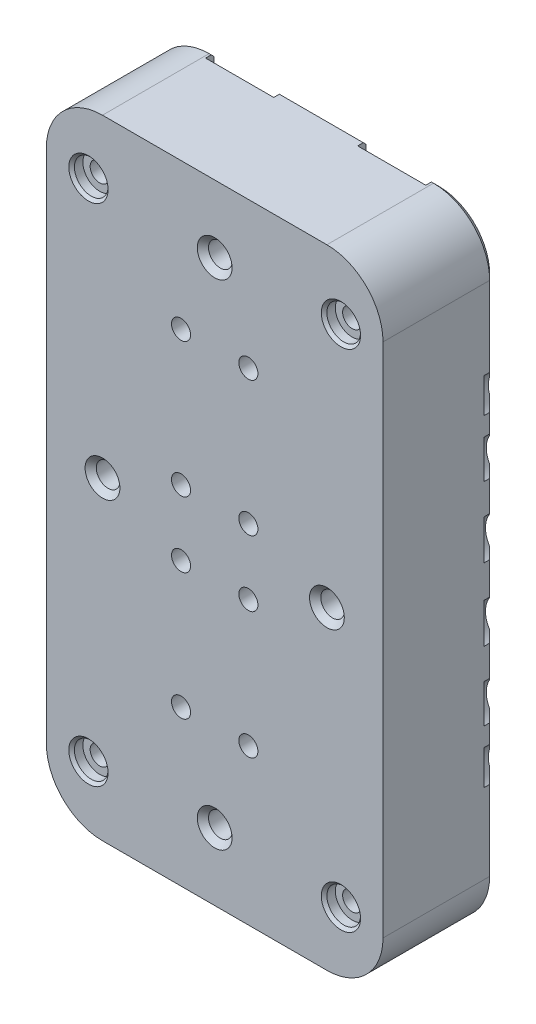
SolidWorks part; units mm, degrees
material "POM 乙缩醛共聚物"
ref_plane "前视" through (0, 0, 0) normal (0, 0, 1) x (1, 0, 0)
ref_plane "上视" through (0, 0, 0) normal (0, 1, 0) x (1, 0, 0)
ref_plane "右视" through (0, 0, 0) normal (1, 0, 0) x (0, 0, -1)
sketch "草图1" plane through (0, 0, 0) normal (0, 0, 1) x (1, 0, 0)
  line L0 (-30, 46) -> (-30, -46)
  line L1 (-20, -56) -> (20, -56)
  line L2 (30, -46) -> (30, 46)
  line L3 (20, 56) -> (-20, 56)
  line L4 (-30, 0) -> (0, 0) construction
  line L5 (0, 56) -> (0, 0) construction
  arc A0 (-30, -46) -> (-20, -56) centre (-20, -46) ccw
  arc A1 (20, -56) -> (30, -46) centre (20, -46) ccw
  arc A2 (30, 46) -> (20, 56) centre (20, 46) ccw
  arc A3 (-30, 46) -> (-20, 56) centre (-20, 46) cw
  dimension "D1" = 10
  dimension "D2" = 112
  dimension "D3" = 60
extrude "凸台-拉伸1" add sketch "草图1" along normal blind 20
hole_wizard "M4 螺纹孔1" positions "草图2" profile "草图3" tap size "M4" standard "AS" end condition through all
sketch "草图2" plane through (0, 0, 20) normal (0, 0, 1) x (1, 0, 0)
  point P0 (22.5, -45)
  point P3 (-22.5, -45)
  point P6 (-22.5, 45)
  point P9 (22.5, 45)
  point P12 (-112.3936, 267.4308)
sketch "草图3" plane through (22.5, -45, 20) normal (1, 0, 0) x (0, -1, 0)
  line L0 (0, 0) -> (0, 20)
  line L1 (0, 20) -> (1.65, 20)
  line L2 (1.65, 20) -> (1.65, 0)
  line L5 (1.65, 0) -> (0, 0)
  line L11 (0, -6.35) -> (0, 107.95) construction
  dimension "通孔螺纹孔钻头直径" = 3.3
  dimension "通孔螺纹孔钻头深度" = 20
cosmetic thread "孔螺蚊线1" parameters "D2"=4
cosmetic thread "孔螺蚊线2" parameters "D2"=4
cosmetic thread "孔螺蚊线6" parameters "D2"=4
cosmetic thread "孔螺蚊线19" parameters "D2"=4
sketch "草图4" plane through (0, 0, 20) normal (0, 0, 1) x (1, 0, 0)
  circle A0 centre (22.5, -45) radius 3
  circle A1 centre (-22.5, -45) radius 3
  circle A2 centre (22.5, 45) radius 3
  circle A3 centre (-22.5, 45) radius 3
  dimension "D1" = 6
  dimension "D2" = 6
  dimension "D3" = 6
  dimension "D4" = 6
extrude "切除-拉伸1" cut sketch "草图4" against normal blind 2
hole_wizard "大小六角凹头盖螺钉柱孔0" positions "草图6" profile "草图7" counterbore size "M3" standard "AS" end condition through all
sketch "草图6" plane through (0, 0, 0) normal (0, 0, -1) x (-1, 0, 0)
  circle A0 centre (22.5, -45) radius 1.65 construction
  point P0 (22.5, 45)
  point P6 (-22.5, -45)
  point P9 (-22.5, 45)
  point P12 (22.5, -45)
sketch "草图7" plane through (-22.5, 45, 0) normal (1, 0, 0) x (0, 1, 0)
  line L0 (0, 0) -> (0, 20)
  line L1 (0, 20) -> (1.7, 20)
  line L3 (1.7, 20) -> (1.7, 4)
  line L4 (1.7, 4) -> (3, 4)
  line L5 (3, 4) -> (3, 0)
  line L7 (3, 0) -> (0, 0)
  line L11 (0, -6.35) -> (0, 107.95) construction
  dimension "通孔孔直径" = 3.4
  dimension "通孔孔深度" = 20
  dimension "柱形沉头孔直径" = 6
  dimension "柱形沉头孔深度" = 4
hole_wizard "大小六角凹头盖螺钉柱孔0" positions "草图10" profile "草图11" counterbore size "M3" standard "AS" end condition through all
sketch "草图10" plane through (0, 0, 0) normal (0, 0, -1) x (-1, 0, 0)
  point P0 (6, 5.95)
  point P7 (-6, 5.95)
  point P13 (6, 29.95)
  point P16 (-6, 29.95)
sketch "草图11" plane through (-6, 5.95, 0) normal (1, 0, 0) x (0, 1, 0)
  line L0 (0, 0) -> (0, 20)
  line L1 (0, 20) -> (1.7, 20)
  line L3 (1.7, 20) -> (1.7, 4)
  line L4 (1.7, 4) -> (3, 4)
  line L5 (3, 4) -> (3, 0)
  line L7 (3, 0) -> (0, 0)
  line L11 (0, -6.35) -> (0, 107.95) construction
  dimension "通孔孔直径" = 3.4
  dimension "通孔孔深度" = 20
  dimension "柱形沉头孔直径" = 6
  dimension "柱形沉头孔深度" = 4
hole_wizard "大小六角凹头盖螺钉柱孔2" positions "草图13" profile "草图14" counterbore size "M3" standard "AS" end condition through all
sketch "草图13" plane through (0, 0, 0) normal (0, 0, -1) x (-1, 0, 0)
  point P0 (-6, -5.75)
  point P3 (6, -5.75)
  point P6 (-6, -28.35)
  point P9 (6, -28.35)
sketch "草图14" plane through (6, -5.75, 0) normal (1, 0, 0) x (0, 1, 0)
  line L0 (0, 0) -> (0, 20)
  line L1 (0, 20) -> (1.7, 20)
  line L3 (1.7, 20) -> (1.7, 4)
  line L4 (1.7, 4) -> (3, 4)
  line L5 (3, 4) -> (3, 0)
  line L7 (3, 0) -> (0, 0)
  line L11 (0, -6.35) -> (0, 107.95) construction
  dimension "通孔孔直径" = 3.4
  dimension "通孔孔深度" = 20
  dimension "柱形沉头孔直径" = 6
  dimension "柱形沉头孔深度" = 4
sketch "草图15" plane through (0, 0, 0) normal (0, 0, 1) x (1, 0, 0)
  line L0 (-20, -56) -> (20, -56) construction
  line L1 (30, -46) -> (30, 46) construction
  line L2 (20, 56) -> (-20, 56) construction
  circle A0 centre (0, -44) radius 6.5
  circle A1 centre (0, 44) radius 6.5
  dimension "D1" = 13
  dimension "D2" = 12
  dimension "D3" = 30
  dimension "D4" = 13
  dimension "D5" = 12
  dimension "D6" = 30
extrude "切除-拉伸3" cut sketch "草图15" along normal blind 8.5
sketch "草图16" plane through (0, 0, 0) normal (0, 0, -1) x (-1, 0, 0)
  circle A0 centre (-20, -0.0001) radius 6.5
  circle A1 centre (20, -0.0001) radius 6.5
  dimension "D1" = 13
  dimension "D2" = 13
  dimension "D3" = 20
  dimension "D4" = 20
extrude "切除-拉伸4" cut sketch "草图16" against normal blind 8.5
hole_wizard "M4 螺纹孔2" positions "草图18" profile "草图19" tap size "M4" standard "AS" end condition through all
sketch "草图18" plane through (0, 0, 8.5) normal (0, 0, -1) x (-1, 0, 0)
  point P0 (-20, -0.0001)
  point P3 (20, -0.0001)
  point P6 (0, 44)
  point P9 (0, -44)
sketch "草图19" plane through (20, -0.0001, 8.5) normal (1, 0, 0) x (0, 1, 0)
  line L0 (0, 0) -> (0, 11.5)
  line L1 (0, 11.5) -> (1.65, 11.5)
  line L2 (1.65, 11.5) -> (1.65, 0)
  line L5 (1.65, 0) -> (0, 0)
  line L11 (0, -6.35) -> (0, 107.95) construction
  dimension "通孔螺纹孔钻头直径" = 3.3
  dimension "通孔螺纹孔钻头深度" = 11.5
cosmetic thread "孔螺蚊线11" parameters "D2"=4
cosmetic thread "孔螺蚊线12" parameters "D2"=4
cosmetic thread "孔螺蚊线13" parameters "D2"=4
cosmetic thread "孔螺蚊线14" parameters "D2"=4
hole_wizard "M5 螺纹孔2" positions "草图20" profile "草图22" tap size "M5" standard "AS"
sketch "草图20" plane through (0, 0, 20) normal (0, 0, 1) x (1, 0, 0)
  point P4 (20, -0.0001)
  point P7 (-20, -0.0001)
  point P10 (0, 44)
  point P13 (0, -44)
sketch "草图22" plane through (20, -0.0001, 20) normal (1, 0, 0) x (0, -1, 0)
  line L0 (0, 0) -> (0, 8.2618)
  line L1 (0, 8.2618) -> (2.1, 7)
  line L2 (2.1, 7) -> (2.1, 0)
  line L5 (2.1, 0) -> (0, 0)
  line L10 (0, 8.2618) -> (-2.1, 7) construction
  line L11 (0, -6.35) -> (0, 107.95) construction
  dimension "螺纹孔钻头直径" = 4.2
  dimension "螺纹孔钻头深度" = 7
  dimension "导头角度" = 118
cosmetic thread "孔螺蚊线15" parameters "D1"=7, "D2"=5
cosmetic thread "孔螺蚊线16" parameters "D1"=7, "D2"=5
cosmetic thread "孔螺蚊线17" parameters "D1"=7, "D2"=5
cosmetic thread "孔螺蚊线18" parameters "D1"=7, "D2"=5
chamfer "倒角1" distance 1 angle 45 8 edges at (30, 0, 0) (27.0711, 53.0711, 0) (27.0711, -53.0711, 0) (0, 56, 0) (0, -56, 0) (-27.0711, 53.0711, 0) (-27.0711, -53.0711, 0) (-30, 0, 0)
sketch "草图23" plane through (0, 0, 0) normal (0, 0, -1) x (-1, 0, 0)
  line L0 (0, 0) -> (33.1344, 0) construction
  line L1 (0, 0) -> (0, -60.1074) construction
  arc A0 (-22.3238, -27.3351) -> (-14.2455, -26.2908) centre (-18.0393, -28.7109) ccw
  arc A1 (-14.2455, -26.2908) -> (-22.3238, -27.3351) centre (-18.53, -24.915) ccw
  arc A2 (14.2455, -26.2908) -> (22.3238, -27.3351) centre (18.53, -24.915) cw
  arc A3 (22.3238, -27.3351) -> (14.2455, -26.2908) centre (18.0393, -28.7109) cw
  arc A4 (22.3238, 27.3351) -> (14.2455, 26.2908) centre (18.0393, 28.7109) ccw
  arc A5 (14.2455, 26.2908) -> (22.3238, 27.3351) centre (18.53, 24.915) ccw
  arc A6 (-14.2455, 26.2908) -> (-22.3238, 27.3351) centre (-18.53, 24.915) cw
  arc A7 (-22.3238, 27.3351) -> (-14.2455, 26.2908) centre (-18.0393, 28.7109) cw
  dimension "D1" = 9
  dimension "D2" = 9
extrude "切除-拉伸5" cut sketch "草图23" against normal blind 2
sketch "草图24" plane through (0, 0, 0) normal (0, 0, -1) x (-1, 0, 0)
  line L0 (20, -56) -> (-20, -56) construction
  line L1 (-7.4791, -56) -> (-19.6265, -56)
  line L2 (-7.4791, -56) -> (-7.4791, -49.7288)
  line L3 (-7.4791, -49.7288) -> (-19.6265, -49.7288)
  line L4 (-19.6265, -56) -> (-19.6265, -49.7288)
  line L5 (0, 0) -> (34.5145, 0) construction
  line L6 (-19.6265, 56) -> (-19.6265, 49.7288)
  line L7 (-14.0278, -53.7288) -> (-11.8778, -53.7288) construction
  line L8 (-7.4791, 49.7288) -> (-19.6265, 49.7288)
  line L9 (-11.4791, -54.1275) -> (-11.4791, -58.5583) construction
  line L10 (-15.6265, -57.3583) -> (-15.6265, -55.3275) construction
  line L11 (-7.4791, 56) -> (-7.4791, 49.7288)
  line L12 (-7.4791, 56) -> (-19.6265, 56)
  line L13 (0, -55) -> (0, 56.9631) construction
  line L14 (-20, -55) -> (20, -55) construction
  line L15 (7.4791, 56) -> (19.6265, 56)
  line L16 (7.4791, 56) -> (7.4791, 49.7288)
  line L17 (7.4791, 49.7288) -> (19.6265, 49.7288)
  line L18 (19.6265, 56) -> (19.6265, 49.7288)
  line L19 (19.6265, -56) -> (19.6265, -49.7288)
  line L20 (7.4791, -49.7288) -> (19.6265, -49.7288)
  line L21 (7.4791, -56) -> (7.4791, -49.7288)
  line L22 (7.4791, -56) -> (19.6265, -56)
  dimension "D1" = 4
  dimension "D2" = 4
  dimension "D3" = 4
extrude "切除-拉伸6" cut sketch "草图24" against normal blind 2
sketch "草图25" plane through (0, 0, 0) normal (0, 0, -1) x (-1, 0, 0)
  line L0 (0, 56) -> (0, -56) construction
  line L2 (20, -56) -> (19.6265, -56) construction
  line L3 (0, 0) -> (37.1883, 0) construction
  line L4 (-7.4791, 56) -> (7.4791, 56) construction
  circle A0 centre (-32.76, 6.44) radius 4.5
  circle A1 centre (-32.91, -18.865) radius 4.5
  circle A2 centre (-33.2748, -28.7109) radius 4.5
  circle A3 centre (33.2748, -28.7109) radius 4.5
  circle A4 centre (32.91, -18.865) radius 4.5
  circle A5 centre (32.76, 6.44) radius 4.5
  circle A6 centre (32.76, -6.44) radius 4.5
  circle A7 centre (32.91, 18.865) radius 4.5
  circle A8 centre (33.2748, 28.7109) radius 4.5
  circle A9 centre (-33.2748, 28.7109) radius 4.5
  circle A10 centre (-32.91, 18.865) radius 4.5
  circle A11 centre (-32.76, -6.44) radius 4.5
  dimension "D1" = 9
  dimension "D2" = 9
  dimension "D3" = 9
extrude "切除-拉伸7" cut sketch "草图25" against normal blind 2
fillet "圆角1" radius 2 8 edges at (7.4791, -49.7288, 1) (19.6265, -49.7288, 1) (19.6265, 49.7288, 1) (7.4791, 49.7288, 1) (-19.6265, 49.7288, 1) (-7.4791, 49.7288, 1) (-7.4791, -49.7288, 1) (-19.6265, -49.7288, 1)
chamfer "倒角2" distance 0.5 angle 45 44 edges at (19.5, 45, 0) (19.5, 45, 4) (-9, 29.95, 0) (3, 29.95, 0) (-19.6265, 53.3644, 0) (-19.0407, 50.3146, 0) (-13.5528, 49.7288, 0) (-8.0648, 50.3146, 0) (-7.4791, 53.3644, 0) (7.4791, 53.3644, 0) (8.0648, 50.3146, 0) (13.5528, 49.7288, 0) (19.0407, 50.3146, 0) (19.6265, 53.3644, 0) (19.1069, 20.4521, 0) (17.4624, 33.1738, 0) (7.4791, -53.3644, 0) (19.6265, -53.3644, 0) (8.0648, -50.3146, 0) (19.0407, -50.3146, 0) (13.5528, -49.7288, 0) (-19.6265, -53.3644, 0) (-7.4791, -53.3644, 0) (-19.0407, -50.3146, 0) (-8.0648, -50.3146, 0) (-13.5528, -49.7288, 0) (-25.5, 45, 0) (-19.1069, 20.4521, 0) (-17.4624, 33.1738, 0) (-26.5, -0.0001, 0) (-9, -5.75, 0) (-9, 5.95, 0) (13.5, -0.0001, 0) (3, 5.95, 0) (3, -5.75, 0) (3, -28.35, 0) (-9, -28.35, 0) (-17.4624, -33.1738, 0) (-19.1069, -20.4521, 0) (17.4624, -33.1738, 0) (19.1069, -20.4521, 0) (19.5, -45, 0) (6.5, -44, 0) (-25.5, -45, 0)
chamfer "倒角3" distance 0.5 angle 45 4 edges at (25.5, 45, 20) (-19.5, 45, 20) (-19.5, -45, 20) (25.5, -45, 20)
chamfer "倒角4" distance 1 angle 45 4 edges at (2.1, 44, 20) (22.1, -0.0001, 20) (-17.9, -0.0001, 20) (2.1, -44, 20)
move or copy body "实体-移动/复制1" [suppressed] bodies to move or copy 116
